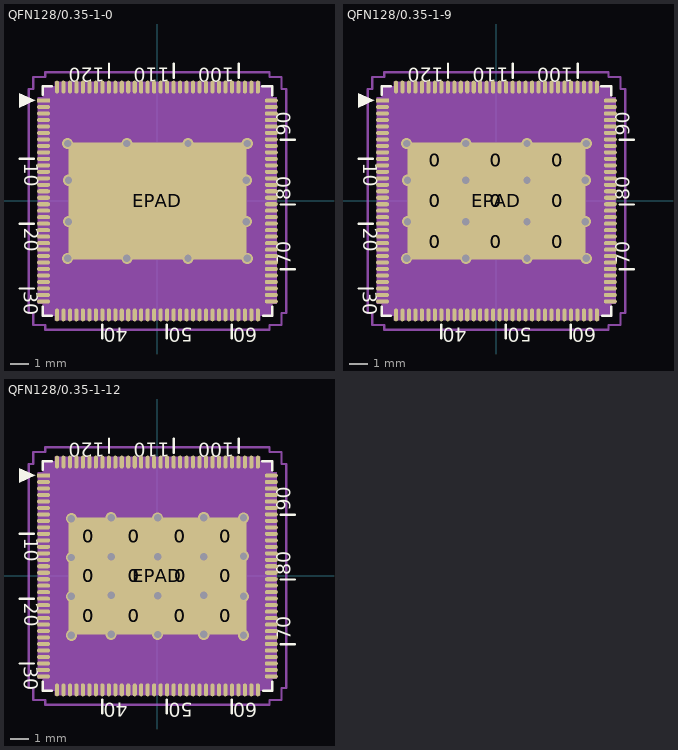
[diagram p0: the footprints below, top view; thin cyan lines are the x and y axes]
# Altium footprint library MISC86372-3.PcbLib: 3 footprints
Each footprint in its own frame and in the unit in brackets; x right, y up, seen from the top. Pads: shape width x height; smd on the part's side, far side on the other; paste and mask are expansions set on the pad; w line width, h text height; cw(c..) or ccw(c..) is an arc to the next point about the centre after c.

## QFN128/0.35-1-0 [mm] "Mstar,TSUMV53RWUT-Z1,18.11.16(19.03.30   reduce extended pad length)"
height 0.9
pads (129):
  rect 0.7x0.22 smd paste-0.02 mask-0.035: 1(-6.151,5.425)
  oval 0.7x0.22 smd paste-0.02 mask-0.035: 2(-6.151,5.075) 3(-6.151,4.725) 4(-6.151,4.375) 5(-6.151,4.025) 6(-6.151,3.675) 7(-6.151,3.325) 8(-6.151,2.975) 9(-6.151,2.625) 10(-6.151,2.275) 11(-6.151,1.925) 12(-6.151,1.575) 13(-6.151,1.225) 14(-6.151,0.875) 15(-6.151,0.525) 16(-6.151,0.175) 17(-6.151,-0.175) 18(-6.151,-0.525) 19(-6.151,-0.875) 20(-6.151,-1.225) 21(-6.151,-1.575) 22(-6.151,-1.925) 23(-6.151,-2.275) 24(-6.151,-2.625) 25(-6.151,-2.975) 26(-6.151,-3.325) 27(-6.151,-3.675) 28(-6.151,-4.025) 29(-6.151,-4.375) 30(-6.151,-4.725) 31(-6.151,-5.075) 32(-6.151,-5.425) 65(6.151,-5.425) 66(6.151,-5.075) 67(6.151,-4.725) 68(6.151,-4.375) 69(6.151,-4.025) 70(6.151,-3.675) 71(6.151,-3.325) 72(6.151,-2.975) 73(6.151,-2.625) 74(6.151,-2.275) 75(6.151,-1.925) 76(6.151,-1.575) 77(6.151,-1.225) 78(6.151,-0.875) 79(6.151,-0.525) 80(6.151,-0.175) 81(6.151,0.175) 82(6.151,0.525) 83(6.151,0.875) 84(6.151,1.225) 85(6.151,1.575) 86(6.151,1.925) 87(6.151,2.275) 88(6.151,2.625) 89(6.151,2.975) 90(6.151,3.325) 91(6.151,3.675) 92(6.151,4.025) 93(6.151,4.375) 94(6.151,4.725) 95(6.151,5.075) 96(6.151,5.425)
  oval 0.22x0.7 smd paste-0.02 mask-0.035: 33(-5.425,-6.151) 34(-5.075,-6.151) 35(-4.725,-6.151) 36(-4.375,-6.151) 37(-4.025,-6.151) 38(-3.675,-6.151) 39(-3.325,-6.151) 40(-2.975,-6.151) 41(-2.625,-6.151) 42(-2.275,-6.151) 43(-1.925,-6.151) 44(-1.575,-6.151) 45(-1.225,-6.151) 46(-0.875,-6.151) 47(-0.525,-6.151) 48(-0.175,-6.151) 49(0.175,-6.151) 50(0.525,-6.151) 51(0.875,-6.151) 52(1.225,-6.151) 53(1.575,-6.151) 54(1.925,-6.151) 55(2.275,-6.151) 56(2.625,-6.151) 57(2.975,-6.151) 58(3.325,-6.151) 59(3.675,-6.151) 60(4.025,-6.151) 61(4.375,-6.151) 62(4.725,-6.151) 63(5.075,-6.151) 64(5.425,-6.151) 97(5.425,6.151) 98(5.075,6.151) 99(4.725,6.151) 100(4.375,6.151) 101(4.025,6.151) 102(3.675,6.151) 103(3.325,6.151) 104(2.975,6.151) 105(2.625,6.151) 106(2.275,6.151) 107(1.925,6.151) 108(1.575,6.151) 109(1.225,6.151) 110(0.875,6.151) 111(0.525,6.151) 112(0.175,6.151) 113(-0.175,6.151) 114(-0.525,6.151) 115(-0.875,6.151) 116(-1.225,6.151) 117(-1.575,6.151) 118(-1.925,6.151) 119(-2.275,6.151) 120(-2.625,6.151) 121(-2.975,6.151) 122(-3.325,6.151) 123(-3.675,6.151) 124(-4.025,6.151) 125(-4.375,6.151) 126(-4.725,6.151) 127(-5.075,6.151) 128(-5.425,6.151)
  rect 9.6x6.3 smd: EPAD(0,0)
via -4.853,-3.103 diameter 0.6 hole 0.4
via 4.853,-3.103 diameter 0.6 hole 0.4
via 4.853,3.103 diameter 0.6 hole 0.4
via -4.853,3.103 diameter 0.6 hole 0.4
via -1.651,3.103 diameter 0.6 hole 0.4
via 4.803,-1.118 diameter 0.6 hole 0.4
via 4.803,1.118 diameter 0.6 hole 0.4
via -4.803,1.118 diameter 0.6 hole 0.4
via -4.803,-1.118 diameter 0.6 hole 0.4
via 1.651,-3.103 diameter 0.6 hole 0.4
via -1.651,-3.103 diameter 0.6 hole 0.4
via 1.651,3.103 diameter 0.6 hole 0.4
Top Overlay:
  region: -6.601,5.435 -7.476,5.821 -7.476,5.049
  lines w0.127: -7.426,-4.723 -6.676,-4.723 ; -7.426,-1.223 -6.676,-1.223 ; -7.426,2.277 -6.676,2.277 ; -6.2,-5.715 -6.2,-6.2 -5.715,-6.2 ; -6.2,5.74 -6.2,6.2 -5.69,6.2 ; -2.989,-7.419 -2.989,-6.669 ; -2.611,6.654 -2.611,7.405 ; 0.511,-7.419 0.511,-6.669 ; 0.889,6.654 0.889,7.405 ; 4.011,-7.419 4.011,-6.669 ; 4.389,6.654 4.389,7.405 ; 5.65,6.2 6.2,6.2 6.2,5.7 ; 5.715,-6.2 6.2,-6.2 6.2,-5.715 ; 6.667,-3.689 7.417,-3.689 ; 6.667,-0.189 7.417,-0.189 ; 6.667,3.311 7.417,3.311
  text "120" at -2.836,7.445 h1.27
  text "110" at 0.664,7.445 h1.27
  text "100" at 4.164,7.445 h1.27
  text "90" at 7.457,3.536 h1.27
  text "80" at 7.457,0.036 h1.27
  text "70" at 7.457,-3.464 h1.27
  text "60" at 5.4,-6.598 h1.27
  text "50" at 1.9,-6.598 h1.27
  text "20" at -7.431,-1.432 h1.27
  text "10" at -7.431,2.068 h1.27
  text "40" at -1.6,-6.598 h1.27
  text "30" at -7.461,-4.875 h1.27
Mechanical 2:
  lines w0.127: -6.95,-6.05 -6.7,-6.05 -6.7,-6.7 -6.05,-6.7 -6.05,-6.95 6.05,-6.95 6.05,-6.7 6.7,-6.7 6.7,-6.05 6.95,-6.05 6.95,6.05 6.7,6.05 6.7,6.7 6.05,6.7 6.05,6.95 -6.05,6.95 -6.05,6.7 -6.7,6.7 -6.7,6.05 -6.95,6.05 -6.95,-6.05
Mechanical 4:
  lines w0.1: -6.15,-6.15 -6.15,6.15 6.15,6.15 6.15,-6.15 -6.15,-6.15
Mechanical 7:
  pour cut-out: -6.45,-5.55 -6.2,-5.55 -6.2,-6.2 -5.55,-6.2 -5.55,-6.45 5.55,-6.45 5.55,-6.2 6.2,-6.2 6.2,-5.55 6.45,-5.55 6.45,5.6 6.2,5.6 6.2,6.2 5.55,6.2 5.55,6.45 -5.55,6.45 -5.55,6.2 -6.2,6.2 -6.2,5.6 -6.45,5.6
3D body: height 0.9, standoff 0, extent -6.2,-6.2 6.2,6.2
3D body: height 0.95, standoff 0.05, extent -5.5,5.15 -5.1,5.55

## QFN128/0.35-1-9 [mm] "Mstar,TSUMV53RWUT-Z1,18.11.16(19.03.30   reduce extended pad length)"
height 0.9
pads (147):
  oct 3x1.9 on Top Solder paste-1: 0(-3.302,-2.21) 0(-3.302,0) 0(-3.302,2.21) 0(0,-2.21) 0(0,0) 0(0,2.21) 0(3.302,-2.21) 0(3.302,0) 0(3.302,2.21)
  oct 3x1.9 on Top Paste paste-1: 0(-3.302,-2.21) 0(-3.302,0) 0(-3.302,2.21) 0(0,-2.21) 0(0,0) 0(0,2.21) 0(3.302,-2.21) 0(3.302,0) 0(3.302,2.21)
  rect 0.7x0.22 smd paste-0.02 mask-0.035: 1(-6.151,5.425)
  oval 0.7x0.22 smd paste-0.02 mask-0.035: 2(-6.151,5.075) 3(-6.151,4.725) 4(-6.151,4.375) 5(-6.151,4.025) 6(-6.151,3.675) 7(-6.151,3.325) 8(-6.151,2.975) 9(-6.151,2.625) 10(-6.151,2.275) 11(-6.151,1.925) 12(-6.151,1.575) 13(-6.151,1.225) 14(-6.151,0.875) 15(-6.151,0.525) 16(-6.151,0.175) 17(-6.151,-0.175) 18(-6.151,-0.525) 19(-6.151,-0.875) 20(-6.151,-1.225) 21(-6.151,-1.575) 22(-6.151,-1.925) 23(-6.151,-2.275) 24(-6.151,-2.625) 25(-6.151,-2.975) 26(-6.151,-3.325) 27(-6.151,-3.675) 28(-6.151,-4.025) 29(-6.151,-4.375) 30(-6.151,-4.725) 31(-6.151,-5.075) 32(-6.151,-5.425) 65(6.151,-5.425) 66(6.151,-5.075) 67(6.151,-4.725) 68(6.151,-4.375) 69(6.151,-4.025) 70(6.151,-3.675) 71(6.151,-3.325) 72(6.151,-2.975) 73(6.151,-2.625) 74(6.151,-2.275) 75(6.151,-1.925) 76(6.151,-1.575) 77(6.151,-1.225) 78(6.151,-0.875) 79(6.151,-0.525) 80(6.151,-0.175) 81(6.151,0.175) 82(6.151,0.525) 83(6.151,0.875) 84(6.151,1.225) 85(6.151,1.575) 86(6.151,1.925) 87(6.151,2.275) 88(6.151,2.625) 89(6.151,2.975) 90(6.151,3.325) 91(6.151,3.675) 92(6.151,4.025) 93(6.151,4.375) 94(6.151,4.725) 95(6.151,5.075) 96(6.151,5.425)
  oval 0.22x0.7 smd paste-0.02 mask-0.035: 33(-5.425,-6.151) 34(-5.075,-6.151) 35(-4.725,-6.151) 36(-4.375,-6.151) 37(-4.025,-6.151) 38(-3.675,-6.151) 39(-3.325,-6.151) 40(-2.975,-6.151) 41(-2.625,-6.151) 42(-2.275,-6.151) 43(-1.925,-6.151) 44(-1.575,-6.151) 45(-1.225,-6.151) 46(-0.875,-6.151) 47(-0.525,-6.151) 48(-0.175,-6.151) 49(0.175,-6.151) 50(0.525,-6.151) 51(0.875,-6.151) 52(1.225,-6.151) 53(1.575,-6.151) 54(1.925,-6.151) 55(2.275,-6.151) 56(2.625,-6.151) 57(2.975,-6.151) 58(3.325,-6.151) 59(3.675,-6.151) 60(4.025,-6.151) 61(4.375,-6.151) 62(4.725,-6.151) 63(5.075,-6.151) 64(5.425,-6.151) 97(5.425,6.151) 98(5.075,6.151) 99(4.725,6.151) 100(4.375,6.151) 101(4.025,6.151) 102(3.675,6.151) 103(3.325,6.151) 104(2.975,6.151) 105(2.625,6.151) 106(2.275,6.151) 107(1.925,6.151) 108(1.575,6.151) 109(1.225,6.151) 110(0.875,6.151) 111(0.525,6.151) 112(0.175,6.151) 113(-0.175,6.151) 114(-0.525,6.151) 115(-0.875,6.151) 116(-1.225,6.151) 117(-1.575,6.151) 118(-1.925,6.151) 119(-2.275,6.151) 120(-2.625,6.151) 121(-2.975,6.151) 122(-3.325,6.151) 123(-3.675,6.151) 124(-4.025,6.151) 125(-4.375,6.151) 126(-4.725,6.151) 127(-5.075,6.151) 128(-5.425,6.151)
  rect 9.6x6.3 smd paste-6 mask-6: EPAD(0,0)
via -4.853,-3.103 diameter 0.6 hole 0.4
via 4.853,-3.103 diameter 0.6 hole 0.4
via 4.853,3.103 diameter 0.6 hole 0.4
via -4.853,3.103 diameter 0.6 hole 0.4
via -1.651,3.103 diameter 0.6 hole 0.4
via 4.803,-1.118 diameter 0.6 hole 0.4
via 4.803,1.118 diameter 0.6 hole 0.4
via -4.803,1.118 diameter 0.6 hole 0.4
via -4.803,-1.118 diameter 0.6 hole 0.4
via 1.651,-3.103 diameter 0.6 hole 0.4
via -1.651,-3.103 diameter 0.6 hole 0.4
via 1.651,3.103 diameter 0.6 hole 0.4
via 1.651,-1.118 diameter 0.6 hole 0.4
via -1.651,-1.118 diameter 0.6 hole 0.4
via -1.651,1.118 diameter 0.6 hole 0.4
via 1.651,1.118 diameter 0.6 hole 0.4
Top Overlay:
  region: -6.601,5.435 -7.476,5.821 -7.476,5.049
  lines w0.127: -7.426,-4.723 -6.676,-4.723 ; -7.426,-1.223 -6.676,-1.223 ; -7.426,2.277 -6.676,2.277 ; -6.2,-5.715 -6.2,-6.2 -5.715,-6.2 ; -6.2,5.74 -6.2,6.2 -5.69,6.2 ; -2.989,-7.419 -2.989,-6.669 ; -2.611,6.654 -2.611,7.405 ; 0.511,-7.419 0.511,-6.669 ; 0.889,6.654 0.889,7.405 ; 4.011,-7.419 4.011,-6.669 ; 4.389,6.654 4.389,7.405 ; 5.65,6.2 6.2,6.2 6.2,5.7 ; 5.715,-6.2 6.2,-6.2 6.2,-5.715 ; 6.667,-3.689 7.417,-3.689 ; 6.667,-0.189 7.417,-0.189 ; 6.667,3.311 7.417,3.311
  text "120" at -2.836,7.445 h1.27
  text "110" at 0.664,7.445 h1.27
  text "100" at 4.164,7.445 h1.27
  text "90" at 7.457,3.536 h1.27
  text "80" at 7.457,0.036 h1.27
  text "70" at 7.457,-3.464 h1.27
  text "60" at 5.4,-6.598 h1.27
  text "50" at 1.9,-6.598 h1.27
  text "20" at -7.431,-1.432 h1.27
  text "10" at -7.431,2.068 h1.27
  text "40" at -1.6,-6.598 h1.27
  text "30" at -7.461,-4.875 h1.27
Mechanical 2:
  lines w0.127: -6.95,-6.05 -6.7,-6.05 -6.7,-6.7 -6.05,-6.7 -6.05,-6.95 6.05,-6.95 6.05,-6.7 6.7,-6.7 6.7,-6.05 6.95,-6.05 6.95,6.05 6.7,6.05 6.7,6.7 6.05,6.7 6.05,6.95 -6.05,6.95 -6.05,6.7 -6.7,6.7 -6.7,6.05 -6.95,6.05 -6.95,-6.05
Mechanical 4:
  lines w0.1: -6.15,-6.15 -6.15,6.15 6.15,6.15 6.15,-6.15 -6.15,-6.15
Mechanical 7:
  pour cut-out: -6.45,-5.55 -6.2,-5.55 -6.2,-6.2 -5.55,-6.2 -5.55,-6.45 5.55,-6.45 5.55,-6.2 6.2,-6.2 6.2,-5.55 6.45,-5.55 6.45,5.6 6.2,5.6 6.2,6.2 5.55,6.2 5.55,6.45 -5.55,6.45 -5.55,6.2 -6.2,6.2 -6.2,5.6 -6.45,5.6
3D body: height 0.9, standoff 0, extent -6.2,-6.2 6.2,6.2
3D body: height 0.95, standoff 0.05, extent -5.5,5.15 -5.1,5.55

## QFN128/0.35-1-12 [mm] "Mstar,TSUMV53RWUT-Z1,18.11.16(19.03.30   reduce extended pad length)"
height 0.9
pads (153):
  oct 2.2x1.9 on Top Solder: 0(-3.7,0) 0(-3.697,-2.145) 0(-3.697,2.145) 0(-1.253,-2.145) 0(-1.253,2.145) 0(-1.25,0) 0(1.247,-2.145) 0(1.247,2.145) 0(1.25,0) 0(3.697,-2.145) 0(3.697,2.145) 0(3.7,0)
  oct 2.2x1.9 on Top Paste: 0(-3.7,0) 0(-3.697,-2.145) 0(-3.697,2.145) 0(-1.253,-2.145) 0(-1.253,2.145) 0(-1.25,0) 0(1.247,-2.145) 0(1.247,2.145) 0(1.25,0) 0(3.697,-2.145) 0(3.697,2.145) 0(3.7,0)
  rect 0.7x0.22 smd paste-0.02 mask-0.035: 1(-6.151,5.425)
  oval 0.7x0.22 smd paste-0.02 mask-0.035: 2(-6.151,5.075) 3(-6.151,4.725) 4(-6.151,4.375) 5(-6.151,4.025) 6(-6.151,3.675) 7(-6.151,3.325) 8(-6.151,2.975) 9(-6.151,2.625) 10(-6.151,2.275) 11(-6.151,1.925) 12(-6.151,1.575) 13(-6.151,1.225) 14(-6.151,0.875) 15(-6.151,0.525) 16(-6.151,0.175) 17(-6.151,-0.175) 18(-6.151,-0.525) 19(-6.151,-0.875) 20(-6.151,-1.225) 21(-6.151,-1.575) 22(-6.151,-1.925) 23(-6.151,-2.275) 24(-6.151,-2.625) 25(-6.151,-2.975) 26(-6.151,-3.325) 27(-6.151,-3.675) 28(-6.151,-4.025) 29(-6.151,-4.375) 30(-6.151,-4.725) 31(-6.151,-5.075) 32(-6.151,-5.425) 65(6.151,-5.425) 66(6.151,-5.075) 67(6.151,-4.725) 68(6.151,-4.375) 69(6.151,-4.025) 70(6.151,-3.675) 71(6.151,-3.325) 72(6.151,-2.975) 73(6.151,-2.625) 74(6.151,-2.275) 75(6.151,-1.925) 76(6.151,-1.575) 77(6.151,-1.225) 78(6.151,-0.875) 79(6.151,-0.525) 80(6.151,-0.175) 81(6.151,0.175) 82(6.151,0.525) 83(6.151,0.875) 84(6.151,1.225) 85(6.151,1.575) 86(6.151,1.925) 87(6.151,2.275) 88(6.151,2.625) 89(6.151,2.975) 90(6.151,3.325) 91(6.151,3.675) 92(6.151,4.025) 93(6.151,4.375) 94(6.151,4.725) 95(6.151,5.075) 96(6.151,5.425)
  oval 0.22x0.7 smd paste-0.02 mask-0.035: 33(-5.425,-6.151) 34(-5.075,-6.151) 35(-4.725,-6.151) 36(-4.375,-6.151) 37(-4.025,-6.151) 38(-3.675,-6.151) 39(-3.325,-6.151) 40(-2.975,-6.151) 41(-2.625,-6.151) 42(-2.275,-6.151) 43(-1.925,-6.151) 44(-1.575,-6.151) 45(-1.225,-6.151) 46(-0.875,-6.151) 47(-0.525,-6.151) 48(-0.175,-6.151) 49(0.175,-6.151) 50(0.525,-6.151) 51(0.875,-6.151) 52(1.225,-6.151) 53(1.575,-6.151) 54(1.925,-6.151) 55(2.275,-6.151) 56(2.625,-6.151) 57(2.975,-6.151) 58(3.325,-6.151) 59(3.675,-6.151) 60(4.025,-6.151) 61(4.375,-6.151) 62(4.725,-6.151) 63(5.075,-6.151) 64(5.425,-6.151) 97(5.425,6.151) 98(5.075,6.151) 99(4.725,6.151) 100(4.375,6.151) 101(4.025,6.151) 102(3.675,6.151) 103(3.325,6.151) 104(2.975,6.151) 105(2.625,6.151) 106(2.275,6.151) 107(1.925,6.151) 108(1.575,6.151) 109(1.225,6.151) 110(0.875,6.151) 111(0.525,6.151) 112(0.175,6.151) 113(-0.175,6.151) 114(-0.525,6.151) 115(-0.875,6.151) 116(-1.225,6.151) 117(-1.575,6.151) 118(-1.925,6.151) 119(-2.275,6.151) 120(-2.625,6.151) 121(-2.975,6.151) 122(-3.325,6.151) 123(-3.675,6.151) 124(-4.025,6.151) 125(-4.375,6.151) 126(-4.725,6.151) 127(-5.075,6.151) 128(-5.425,6.151)
  rect 9.6x6.3 smd paste-6 mask-6: EPAD(0,0)
via 4.65,3.138 diameter 0.6 hole 0.4
via 0.012,3.138 diameter 0.6 hole 0.4
via 0.012,-3.162 diameter 0.6 hole 0.4
via 0.012,-1.062 diameter 0.6 hole 0.4
via 0.012,1.038 diameter 0.6 hole 0.4
via -4.65,3.1 diameter 0.6 hole 0.4
via -4.65,1 diameter 0.6 hole 0.4
via -4.65,-1.1 diameter 0.6 hole 0.4
via -4.65,-3.2 diameter 0.6 hole 0.4
via 4.65,-3.2 diameter 0.6 hole 0.4
via 4.65,-1.1 diameter 0.6 hole 0.4
via -2.5,3.15 diameter 0.6 hole 0.4
via 4.65,1.075 diameter 0.6 hole 0.4
via 2.5,3.15 diameter 0.6 hole 0.4
via 2.5,-3.15 diameter 0.6 hole 0.4
via -2.5,-3.15 diameter 0.6 hole 0.4
via -2.5,1.05 diameter 0.6 hole 0.4
via -2.5,-1.05 diameter 0.6 hole 0.4
via 2.5,-1.05 diameter 0.6 hole 0.4
via 2.5,1.05 diameter 0.6 hole 0.4
Top Overlay:
  region: -6.601,5.435 -7.476,5.821 -7.476,5.049
  lines w0.127: -7.426,-4.723 -6.676,-4.723 ; -7.426,-1.223 -6.676,-1.223 ; -7.426,2.277 -6.676,2.277 ; -6.2,-5.715 -6.2,-6.2 -5.715,-6.2 ; -6.2,5.74 -6.2,6.2 -5.69,6.2 ; -2.989,-7.419 -2.989,-6.669 ; -2.611,6.654 -2.611,7.405 ; 0.511,-7.419 0.511,-6.669 ; 0.889,6.654 0.889,7.405 ; 4.011,-7.419 4.011,-6.669 ; 4.389,6.654 4.389,7.405 ; 5.65,6.2 6.2,6.2 6.2,5.7 ; 5.715,-6.2 6.2,-6.2 6.2,-5.715 ; 6.667,-3.689 7.417,-3.689 ; 6.667,-0.189 7.417,-0.189 ; 6.667,3.311 7.417,3.311
  text "30" at -7.461,-4.875 h1.27
  text "40" at -1.6,-6.598 h1.27
  text "10" at -7.431,2.068 h1.27
  text "20" at -7.431,-1.432 h1.27
  text "50" at 1.9,-6.598 h1.27
  text "60" at 5.4,-6.598 h1.27
  text "70" at 7.457,-3.464 h1.27
  text "80" at 7.457,0.036 h1.27
  text "90" at 7.457,3.536 h1.27
  text "100" at 4.164,7.445 h1.27
  text "110" at 0.664,7.445 h1.27
  text "120" at -2.836,7.445 h1.27
Mechanical 2:
  lines w0.127: -6.95,-6.05 -6.95,6.05 -6.7,6.05 -6.7,6.7 -6.05,6.7 -6.05,6.95 6.05,6.95 6.05,6.7 6.7,6.7 6.7,6.05 6.95,6.05 6.95,-6.05 6.7,-6.05 6.7,-6.7 6.05,-6.7 6.05,-6.95 -6.05,-6.95 -6.05,-6.7 -6.7,-6.7 -6.7,-6.05 -6.95,-6.05
Mechanical 4:
  lines w0.1: -6.15,-6.15 6.15,-6.15 6.15,6.15 -6.15,6.15 -6.15,-6.15
Mechanical 7:
  pour cut-out: -6.45,-5.55 -6.2,-5.55 -6.2,-6.2 -5.55,-6.2 -5.55,-6.45 5.55,-6.45 5.55,-6.2 6.2,-6.2 6.2,-5.55 6.45,-5.55 6.45,5.6 6.2,5.6 6.2,6.2 5.55,6.2 5.55,6.45 -5.55,6.45 -5.55,6.2 -6.2,6.2 -6.2,5.6 -6.45,5.6
3D body: height 0.95, standoff 0.05, extent -5.5,5.15 -5.1,5.55
3D body: height 0.9, standoff 0, extent -6.2,-6.2 6.2,6.2